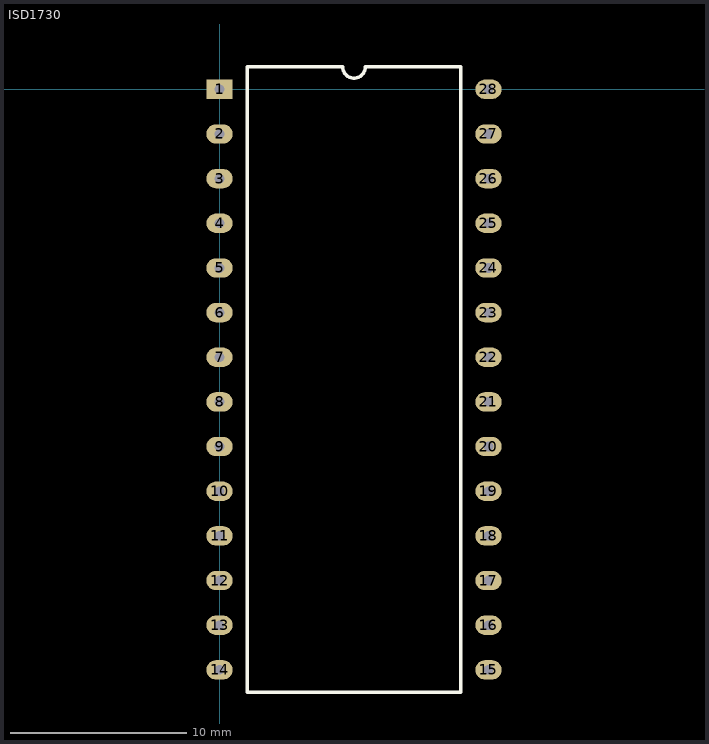
[diagram p0: the footprints below, top view; thin cyan lines are the x and y axes]
# Altium footprint library MISC86338-4.PcbLib: 2 footprints
Each footprint in its own frame and in the unit in brackets; x right, y up, seen from the top. Pads: shape width x height; smd on the part's side, far side on the other; paste and mask are expansions set on the pad; w line width, h text height; cw(c..) or ccw(c..) is an arc to the next point about the centre after c.

## ISD1730 [mm]
pads (28):
  rect 1.5x1.1 hole 0.55: 1(0,0)
  oval 1.5x1.1 hole 0.55: 2(0,-2.54) 3(0,-5.08) 4(0,-7.62) 5(0,-10.16) 6(0,-12.7) 7(0,-15.24) 8(0,-17.78) 9(0,-20.32) 10(0,-22.86) 11(0,-25.4) 12(0,-27.94) 13(0,-30.48) 14(0,-33.02) 15(15.3,-33.02) 16(15.3,-30.48) 17(15.3,-27.94) 18(15.3,-25.4) 19(15.3,-22.86) 20(15.3,-20.32) 21(15.3,-17.78) 22(15.3,-15.24) 23(15.3,-12.7) 24(15.3,-10.16) 25(15.3,-7.62) 26(15.3,-5.08) 27(15.3,-2.54) 28(15.3,0)
Top Overlay:
  lines w0.2: 1.585,-34.29 1.585,1.27 7.015,1.27 ccw(c7.65,1.27) 8.285,1.27 13.715,1.27 13.715,-34.29 1.585,-34.29

## PCBComponent_1 [mm]